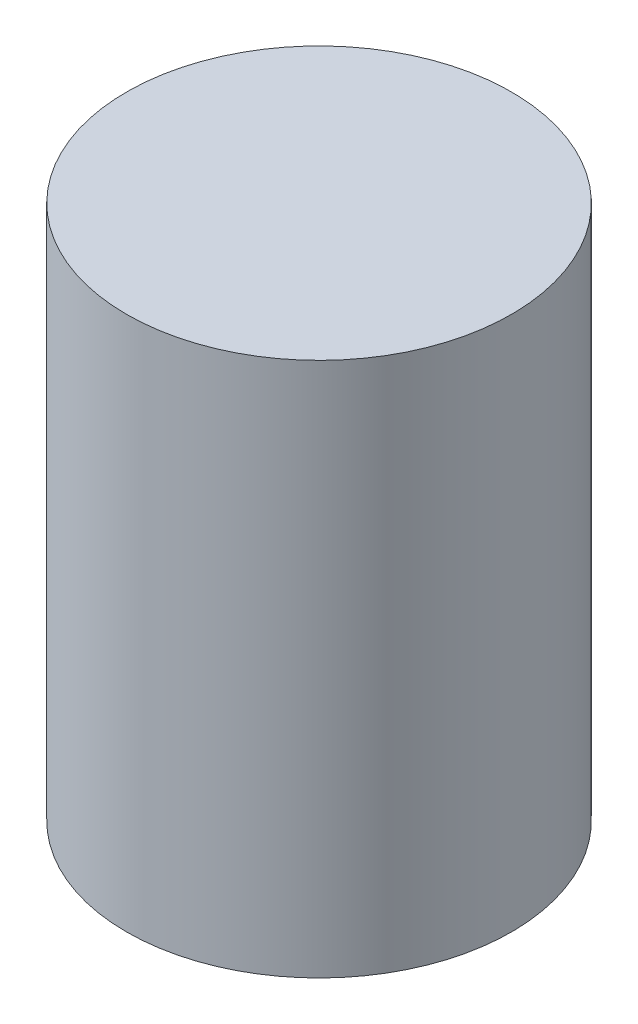
SolidWorks part; units mm, degrees
material "6061"
ref_plane "前视基准面" through (0, 0, 0) normal (0, 0, 1) x (1, 0, 0)
ref_plane "上视基准面" through (0, 0, 0) normal (0, 1, 0) x (1, 0, 0)
ref_plane "右视基准面" through (0, 0, 0) normal (1, 0, 0) x (0, 0, -1)
sketch "草图1" plane through (0, 0, 0) normal (0, 1, 0) x (1, 0, 0)
  circle A0 centre (0, 0) radius 9
  dimension "D1" = 18
extrude "凸台-拉伸1" add sketch "草图1" along normal mid plane 25
